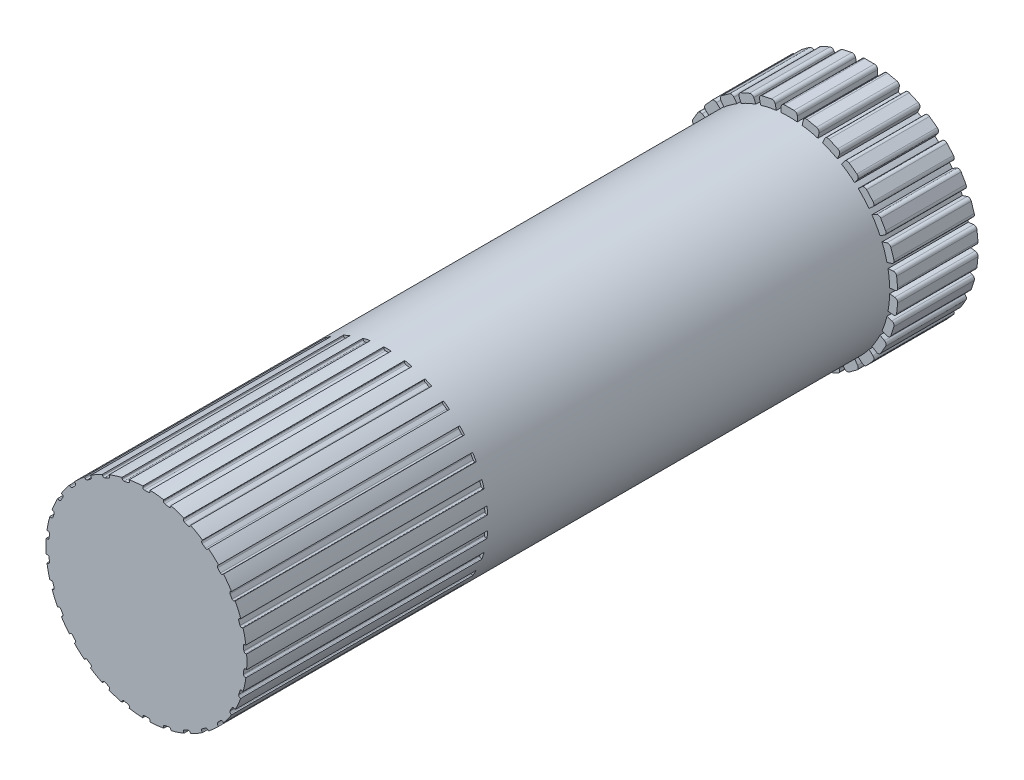
SolidWorks part; units mm, degrees
ref_plane "Front Plane" through (0, 0, 0) normal (0, 0, 1) x (1, 0, 0)
ref_plane "Top Plane" through (0, 0, 0) normal (0, 1, 0) x (1, 0, 0)
ref_plane "Right Plane" through (0, 0, 0) normal (1, 0, 0) x (0, 0, -1)
sketch "Sketch1" plane through (0, 0, 0) normal (0, 0, 1) x (1, 0, 0)
  circle A0 centre (0, 0) radius 12.5
  dimension "D1" = 25
extrude "Boss-Extrude1" add sketch "Sketch1" along normal blind 90
sketch "Sketch3" plane through (0, 0, 90) normal (0, 0, 1) x (1, 0, 0)
  line L0 (0, 0) -> (0, 17.6244) construction
  line L2 (-0.4576, 12.8402) -> (0.4576, 12.8402)
  line L3 (-0.4576, 12.8402) -> (-0.4576, 12.3598)
  line L4 (-0.2576, 12.1598) -> (0.2576, 12.1598)
  line L5 (0.4576, 12.8402) -> (0.4576, 12.3598)
  line L6 (-0.4576, 12.8402) -> (0.4576, 12.1598) construction
  line L7 (-0.4576, 12.1598) -> (0.4576, 12.8402) construction
  circle A0 centre (0, 0) radius 12.5 construction
  arc A1 (0.2576, 12.1598) -> (0.4576, 12.3598) centre (0.2576, 12.3598) ccw
  arc A2 (-0.4576, 12.3598) -> (-0.2576, 12.1598) centre (-0.2576, 12.3598) ccw
  point P3 (0, 12.5)
  dimension "D1" = 0.2
extrude "Cut-Extrude1" cut sketch "Sketch3" against normal blind 30
pattern_circular "CirPattern1" count 30 over 360 about axis through (0, 0, 0) along (0, 0, 1) of "Cut-Extrude1"
sketch "Sketch6" plane through (0, 0, 0) normal (0, 0, -1) x (-1, 0, 0)
  line L0 (0, 0) -> (0, 18.9975) construction
  line L2 (-0.6, 13.5) -> (0.6, 13.5)
  line L3 (-1, 13.1) -> (-1, 11.9)
  line L4 (-0.6, 11.5) -> (0.6, 11.5)
  line L5 (1, 13.1) -> (1, 11.9)
  line L6 (-1, 13.5) -> (1, 11.5) construction
  line L7 (-1, 11.5) -> (1, 13.5) construction
  circle A0 centre (0, 0) radius 12.5 construction
  arc A1 (0.6, 11.5) -> (1, 11.9) centre (0.6, 11.9) ccw
  arc A2 (-1, 11.9) -> (-0.6, 11.5) centre (-0.6, 11.9) ccw
  arc A3 (1, 13.1) -> (0.6, 13.5) centre (0.6, 13.1) ccw
  arc A4 (-1, 13.1) -> (-0.6, 13.5) centre (-0.6, 13.1) cw
  point P3 (0, 12.5)
  dimension "D2" = 0.4
  dimension "D3" = 0.4
  dimension "D1" = 2
extrude "Boss-Extrude2" add sketch "Sketch6" against normal blind 10
pattern_circular "CirPattern4" count 30 over 360 about axis through (0, 0, 0) along (0, 0, 1) of "Boss-Extrude2"
